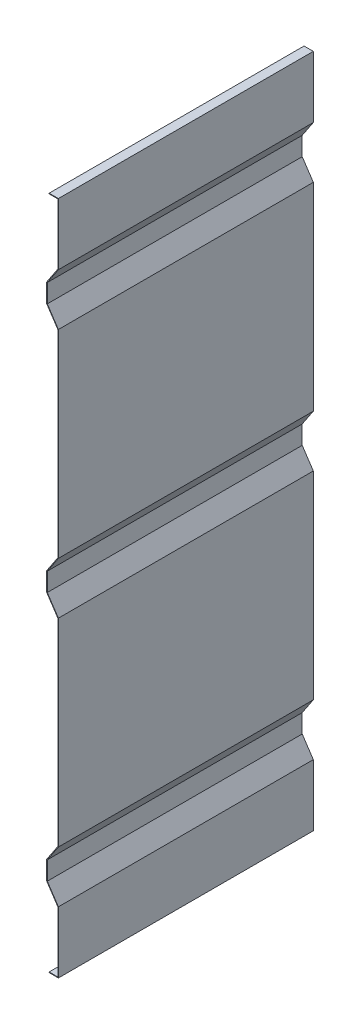
from build123d import *

# Parameters (mm, degrees)
EXTRUDE_THIN1_DEPTH = 413.5


with BuildPart() as part:
    # Sketch1 → Extrude-Thin1 (new, symmetric)
    with BuildSketch(Plane.XY):
        Polygon((-30, -1095), (0, -1095), (0, -895), (-36, -841), (-36, -781), (0, -727), (0, -84), (-36, -30), (-36, 30), (0, 84), (0, 727), (-36, 781), (-36, 841), (0, 895), (0, 1095), (-30, 1095), (-30, 1093), (-2, 1093), (-2, 895.605551275), (-38, 841.605551275), (-38, 780.394448725), (-2, 726.394448725), (-2, 84.605551275), (-38, 30.605551275), (-38, -30.605551275), (-2, -84.605551275), (-2, -726.394448725), (-38, -780.394448725), (-38, -841.605551275), (-2, -895.605551275), (-2, -1093), (-30, -1093), align=None)
    extrude(amount=EXTRUDE_THIN1_DEPTH, both=True)


solid = part.part
